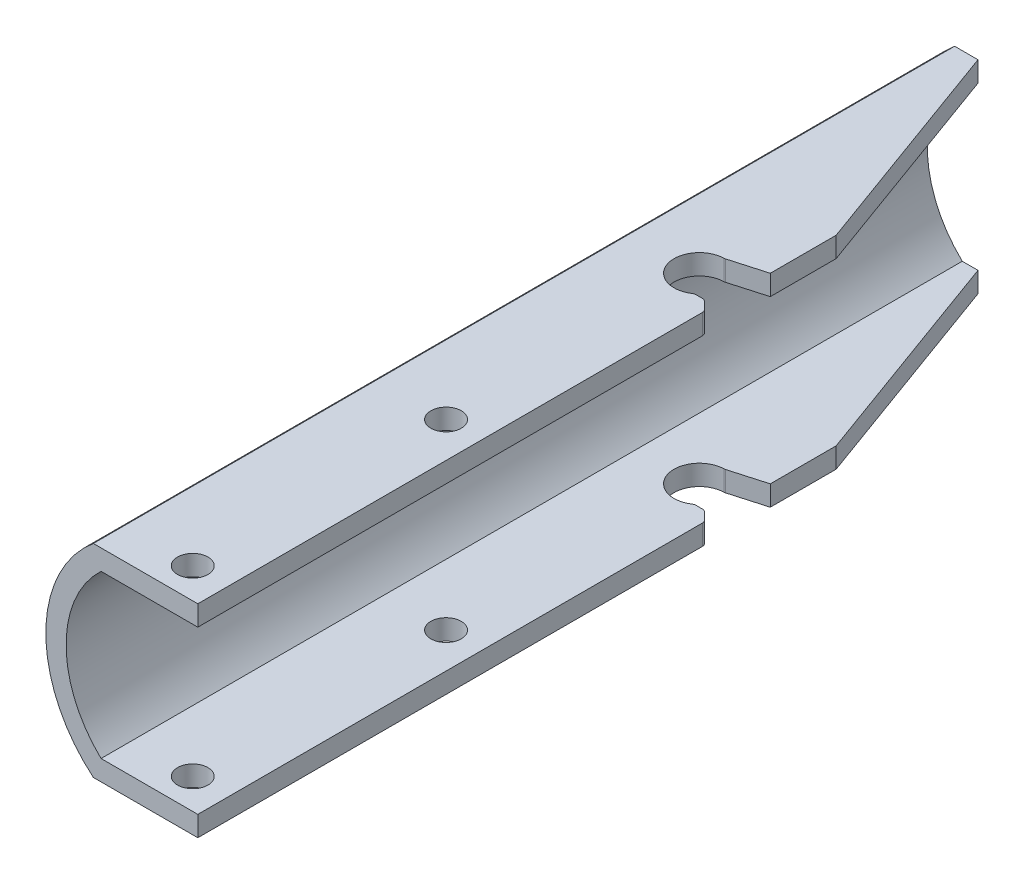
from build123d import *

# Parameters (mm, degrees)
BOSS_EXTRUDE1_DEPTH = 85
SKETCH2_R           = 1.5
CUT_EXTRUDE1_DEPTH  = 89.283633817
CUT_EXTRUDE2_DEPTH  = 89.283633817
FILLET1_R           = 0.5
FILLET2_R           = 0.5


with BuildPart() as part:
    # Sketch1 → Boss-Extrude1 (new body)
    with BuildSketch(Plane.XY):
        with BuildLine():
            Line((-8.306623863, 10), (2, 10))
            Line((2, 10), (2, 8))
            Line((2, 8), (-7.549834435, 8))
            ThreePointArc((-7.549834435, 8), (-11, 0), (-7.549834435, -8))
            Line((-7.549834435, -8), (2, -8))
            Line((2, -8), (2, -10))
            Line((2, -10), (-8.306623863, -10))
            ThreePointArc((-8.306623863, -10), (-13, 0), (-8.306623863, 10))
        make_face()
    extrude(amount=BOSS_EXTRUDE1_DEPTH)

    # Sketch2 → Cut-Extrude1 (cut, through all)
    with BuildSketch(Plane(origin=(0, -10, 0), x_dir=(-1, 0, 0), z_dir=(0, -1, 0))):
        with Locations(Location((1.5, -82, 0), (0, 0, 90))):
            Circle(SKETCH2_R)
        with Locations(Location((1.5, -57, 0), (0, 0, 90))):
            Circle(SKETCH2_R)
        Polygon((-2, -22), (6, 0), (-2, 0), align=None)
    extrude(amount=-CUT_EXTRUDE1_DEPTH, mode=Mode.SUBTRACT)

    # Sketch3 → Cut-Extrude2 (cut, through all)
    with BuildSketch(Plane(origin=(0, -10, 0), x_dir=(-1, 0, 0), z_dir=(0, -1, 0))):
        with BuildLine():
            Line((-2, -28.5), (-2, -35))
            Line((-2, -35), (-1, -34))
            Line((-1, -34), (0, -34))
            ThreePointArc((0, -34), (3.871708245, -32.790569415), (1.5, -29.5))
            Line((1.5, -29.5), (-2, -28.5))
        make_face()
    extrude(amount=-CUT_EXTRUDE2_DEPTH, mode=Mode.SUBTRACT)

    # Fillet1
    fillet1_edges = [part.edges().sort_by_distance(p)[0] for p in [
        (1, -9, 34),
        (1, 9, 34),
        (2, -9, 35),
        (2, 9, 35),
        (0, -9, 34),
        (0, 9, 34),
    ]]
    fillet(fillet1_edges, radius=FILLET1_R)

    # Fillet2
    fillet2_edges = [part.edges().sort_by_distance(p)[0] for p in [
        (-1.5, -9, 29.5),
        (-1.5, 9, 29.5),
    ]]
    fillet(fillet2_edges, radius=FILLET2_R)


solid = part.part
